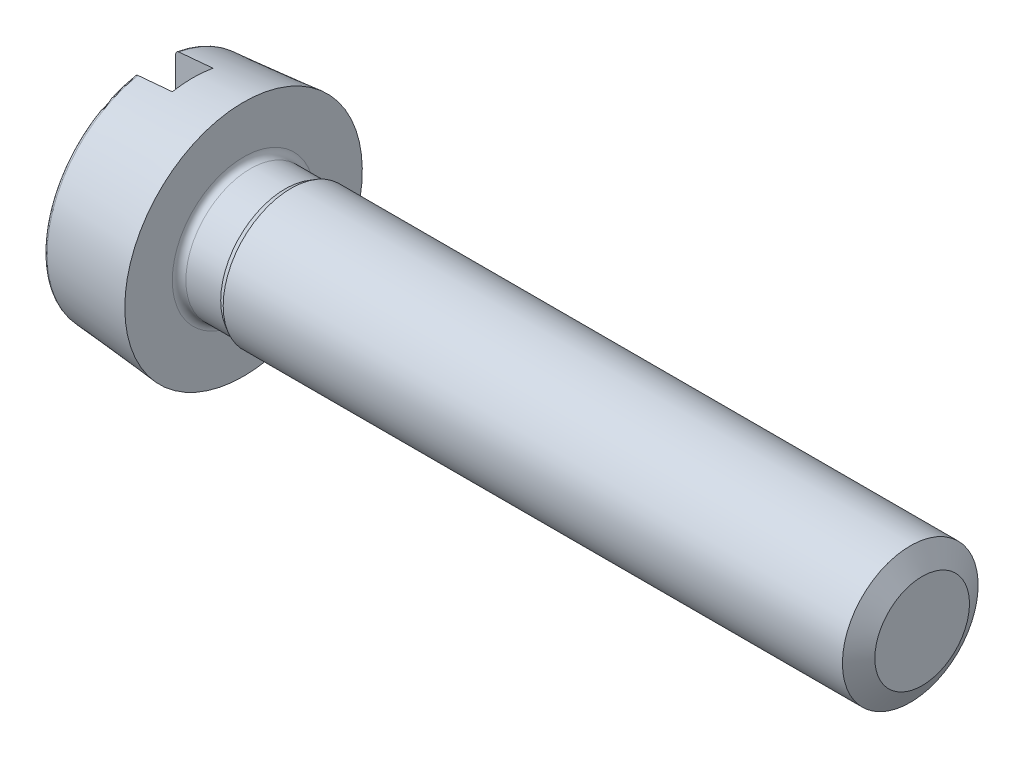
from build123d import *

# Parameters (mm, degrees)
CUT_EXTRUDE1_DEPTH = 1.1


with BuildPart() as part:
    # Sketch1 → Base-Revolve (revolve)
    with BuildSketch(Plane.XY, mode=Mode.PRIVATE) as base_revolve_sk:
        with BuildLine():
            Line((0, 0), (0, 3.180896357))
            ThreePointArc((0, 3.180896357), (0.026272266, 3.248455378), (0.091284426, 3.280515827))
            Line((0.091284426, 3.280515827), (2.6, 3.5))
            Line((2.6, 3.5), (2.6, 2.1))
            ThreePointArc((2.6, 2.1), (2.658578644, 1.958578644), (2.8, 1.9))
            Line((2.8, 1.9), (3.826794919, 1.9))
            Line((3.826794919, 1.9), (4, 2))
            Line((4, 2), (22.6, 2))
            Line((22.6, 2), (22.6, 0))
            Line((22.6, 0), (0, 0))
        make_face()
    revolve(base_revolve_sk.sketch.rotate(Axis((0, 0, 0), (1, 0, 0)), 90), axis=Axis((0, 0, 0), (1, 0, 0)))

    # Sketch2 → Cut-Extrude1 (cut)
    with BuildSketch(Plane.ZY):
        with BuildLine():
            Line((0.6, 3.44818793), (0.6, -3.44818793))
            ThreePointArc((0.6, -3.44818793), (0, -3.5), (-0.6, -3.44818793))
            Line((-0.6, -3.44818793), (-0.6, 3.44818793))
            ThreePointArc((-0.6, 3.44818793), (0, 3.5), (0.6, 3.44818793))
        make_face()
    extrude(amount=-CUT_EXTRUDE1_DEPTH, mode=Mode.SUBTRACT)

    # Sketch3 → Cut-Revolve1 (revolve, cut)
    with BuildSketch(Plane(origin=(0, 0, 0), x_dir=(1, 0, 0), z_dir=(0, 1, 0)), mode=Mode.PRIVATE) as cut_revolve1_sk:
        Polygon((22.250010267, 2), (22.949989733, 2), (22.6, 1.3938), align=None)
    revolve(cut_revolve1_sk.sketch.rotate(Axis((0, 0, 0), (1, 0, 0)), 180), axis=Axis((0, 0, 0), (1, 0, 0)), mode=Mode.SUBTRACT)


solid = part.part
